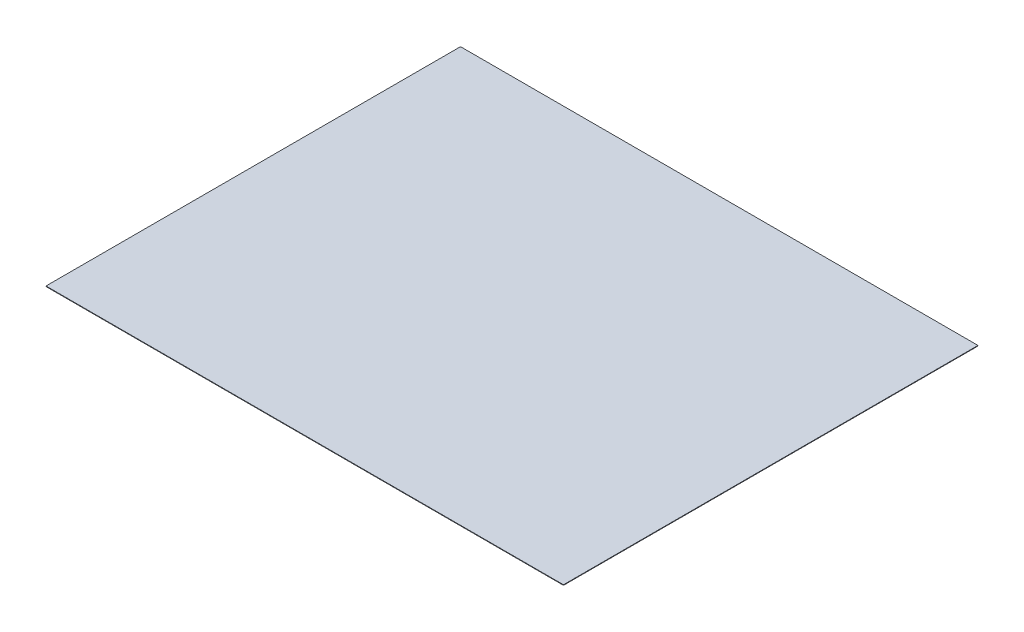
from build123d import *

# Parameters (mm, degrees)
SKETCH1_W           = 1000
SKETCH1_H           = 801
BOSS_EXTRUDE1_DEPTH = 1


with BuildPart() as part:
    # Sketch1 → Boss-Extrude1 (new body)
    with BuildSketch(Plane(origin=(0, 0, 0), x_dir=(1, 0, 0), z_dir=(0, 1, 0))):
        Rectangle(SKETCH1_W, SKETCH1_H)
    extrude(amount=BOSS_EXTRUDE1_DEPTH)


solid = part.part
